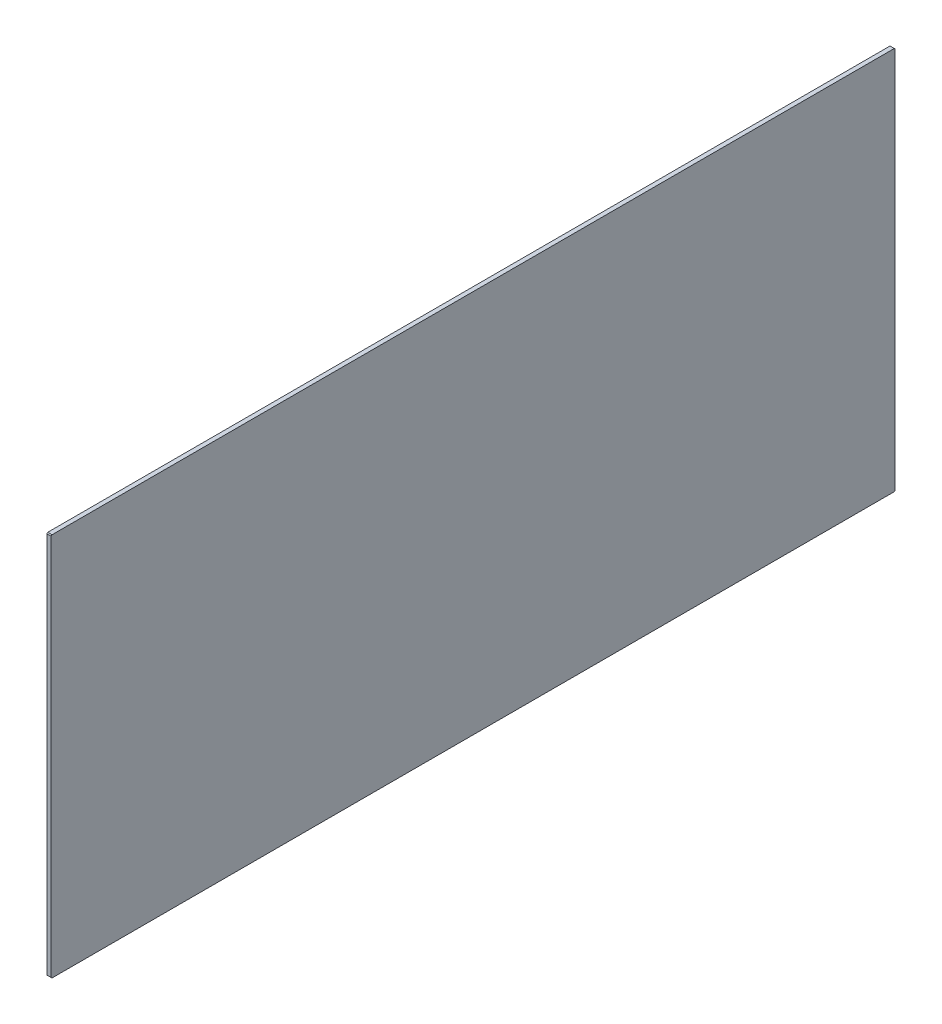
SolidWorks part; units mm, degrees
material "C-玻璃纤维"
ref_plane "前视基准面" through (0, 0, 0) normal (0, 0, 1) x (1, 0, 0)
ref_plane "上视基准面" through (0, 0, 0) normal (0, 1, 0) x (1, 0, 0)
ref_plane "右视基准面" through (0, 0, 0) normal (1, 0, 0) x (0, 0, -1)
sketch "草图2" plane through (0, 0, 0) normal (1, 0, 0) x (0, 0, -1)
  line L1 (-492.5, 224) -> (492.5, 224)
  line L2 (-492.5, 224) -> (-492.5, -224)
  line L3 (-492.5, -224) -> (492.5, -224)
  line L4 (492.5, 224) -> (492.5, -224)
  line L5 (-492.5, 224) -> (492.5, -224) construction
  line L6 (-492.5, -224) -> (492.5, 224) construction
  point P0 (0, 0)
  dimension "D1" = 985
  dimension "D2" = 448
extrude "凸台-拉伸1" add sketch "草图2" along normal blind 5 separate body
chamfer "倒角1" distance 1 angle 45 4 edges at (2.5, 224, 492.5) (2.5, -224, 492.5) (2.5, -224, -492.5) (2.5, 224, -492.5)
